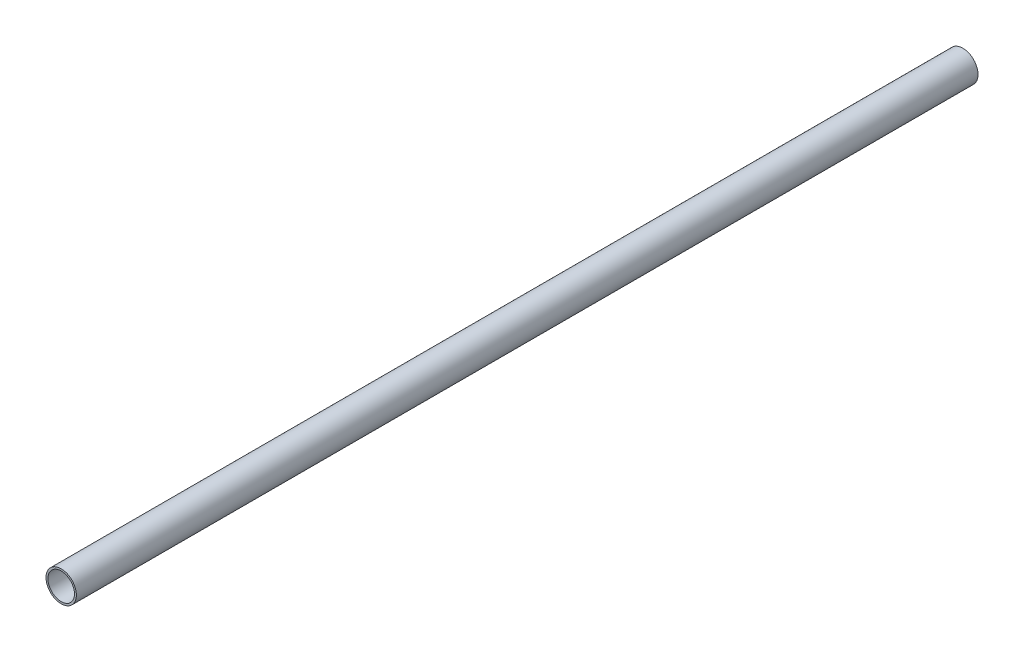
from build123d import *

# Parameters (mm, degrees)
SKETCH_1_R      = 16
SKETCH_1_R_2    = 14
EXTRUDE_1_DEPTH = 475


with BuildPart() as part:
    # 草图1 → 凸台-拉伸1 (new, symmetric)
    with BuildSketch(Plane.XY):
        with Locations(Location((0, 0, 0), (0, 0, 180))):
            Circle(SKETCH_1_R)
        with Locations(Location((0, 0, 0), (0, 0, 180))):
            Circle(SKETCH_1_R_2, mode=Mode.SUBTRACT)
    extrude(amount=EXTRUDE_1_DEPTH, both=True)


solid = part.part
